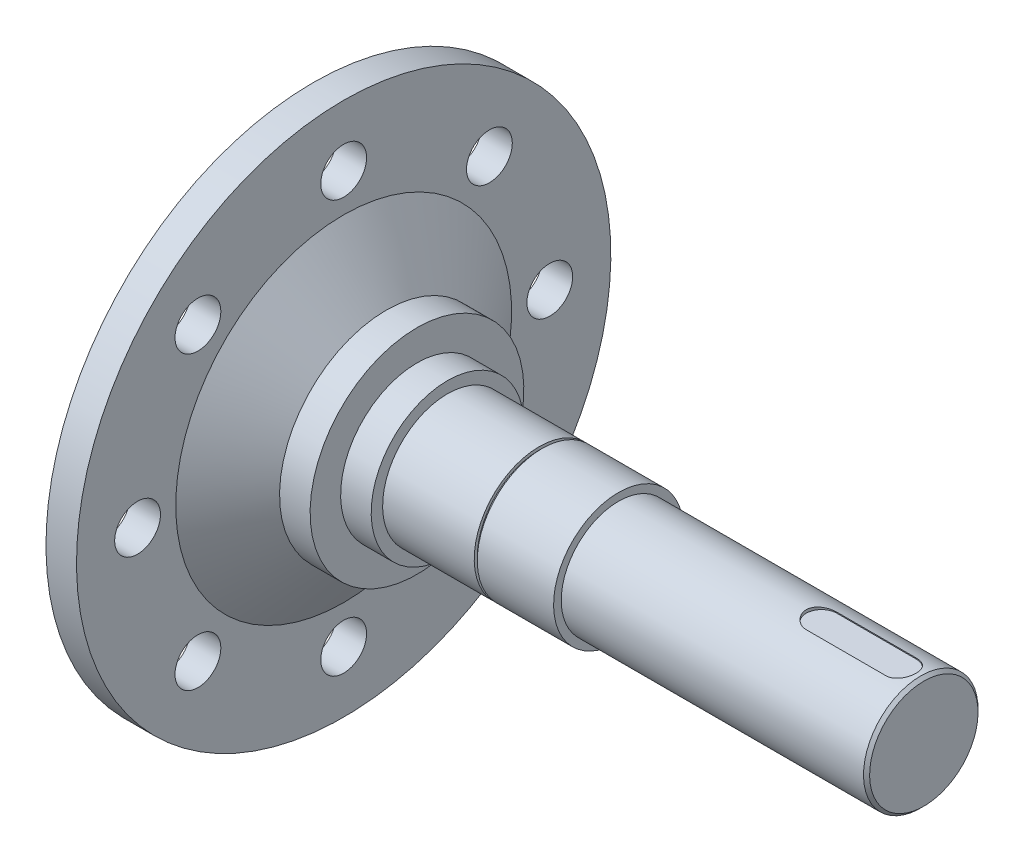
from build123d import *

# Parameters (mm, degrees)
SKETCH_2_R          = 45
CUT_EXTRUDE_1_DEPTH = 30
CHAMFER_1_SIZE      = 10
CUT_EXTRUDE_2_DEPTH = 2
CHAMFER_2_SIZE      = 2
SKETCH_4_R          = 15
CUT_EXTRUDE_3_DEPTH = 50


with BuildPart() as part:
    # 草图1 → 旋转1 (revolve)
    with BuildSketch(Plane.XY):
        Polygon((0, 0), (0, 175), (20, 175), (20, 110), (48.008301528, 70), (68.008301528, 70), (68.008301528, 50), (88.008301528, 50), (88.008301528, 42.5), (148, 42.5), (148, 40.5), (150, 40.5), (150, 42.5), (200, 42.5), (200, 37.5), (400, 37.5), (400, 0), align=None)
    revolve(axis=Axis((400, 0, 0), (-1, 0, 0)))

    # 草图2 → 切除-拉伸1 (cut)
    with BuildSketch(Plane.ZY):
        with Locations(Location((0, 0, 0), (0, 0, 270))):
            Circle(SKETCH_2_R)
    extrude(amount=-CUT_EXTRUDE_1_DEPTH, mode=Mode.SUBTRACT)

    # 倒角1
    chamfer_1_edges = [part.edges().sort_by_distance(p)[0] for p in [
        (0, 45, 0),
    ]]
    chamfer(chamfer_1_edges, length=CHAMFER_1_SIZE)

    # 草图3 → 切除-拉伸2 (cut)
    with BuildSketch(Plane(origin=(0, 37.5, 0), x_dir=(1, 0, 0), z_dir=(0, 1, 0))):
        with BuildLine():
            Line((333, 10), (385, 10))
            ThreePointArc((385, 10), (395, 0), (385, -10))
            Line((385, -10), (333, -10))
            ThreePointArc((333, -10), (323, 0), (333, 10))
        make_face()
    extrude(amount=-CUT_EXTRUDE_2_DEPTH, mode=Mode.SUBTRACT)

    # 倒角2
    chamfer_2_edges = [part.edges().sort_by_distance(p)[0] for p in [
        (400, -37.5, 0),
    ]]
    chamfer(chamfer_2_edges, length=CHAMFER_2_SIZE)

    # 草图4 → 切除-拉伸3 (cut)
    with BuildSketch(Plane.ZY):
        with Locations(Location((0, 135, 0), (0, 0, 270))):
            Circle(SKETCH_4_R)
        with Locations(Location((95.45941546, 95.45941546, 0), (0, 0, 270))):
            Circle(SKETCH_4_R)
        with Locations(Location((135, 0, 0), (0, 0, 270))):
            Circle(SKETCH_4_R)
        with Locations(Location((95.45941546, -95.45941546, 0), (0, 0, 270))):
            Circle(SKETCH_4_R)
        with Locations(Location((0, -135, 0), (0, 0, 270))):
            Circle(SKETCH_4_R)
        with Locations(Location((-95.45941546, -95.45941546, 0), (0, 0, 270))):
            Circle(SKETCH_4_R)
        with Locations(Location((-135, 0, 0), (0, 0, 270))):
            Circle(SKETCH_4_R)
        with Locations(Location((-95.45941546, 95.45941546, 0), (0, 0, 270))):
            Circle(SKETCH_4_R)
    extrude(amount=-CUT_EXTRUDE_3_DEPTH, mode=Mode.SUBTRACT)


solid = part.part
